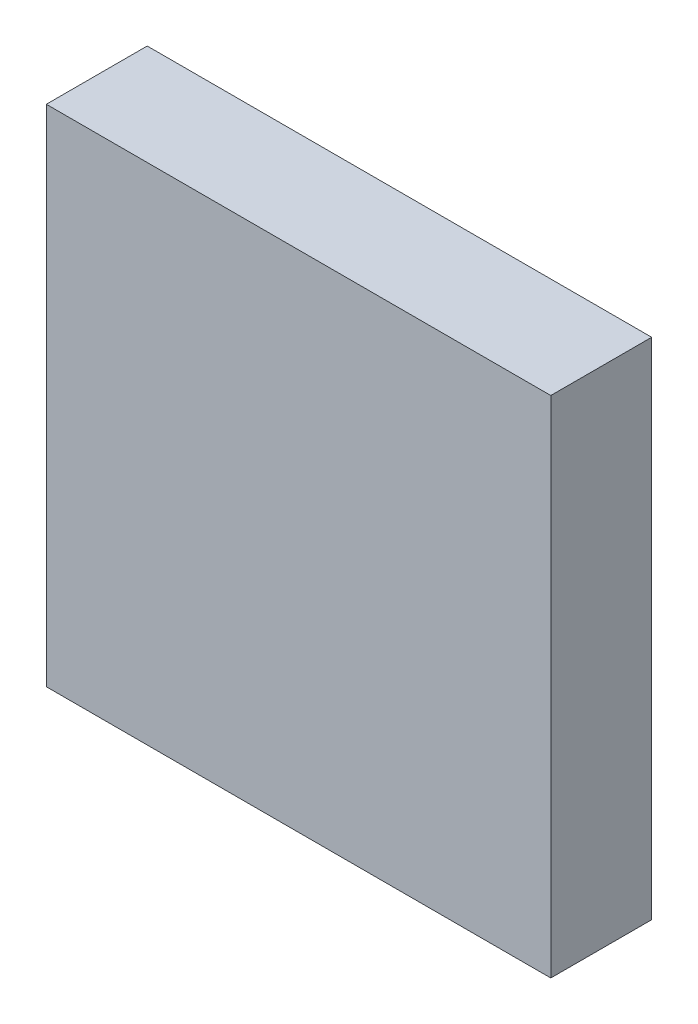
SolidWorks part; units mm, degrees
material "Q235"
ref_plane "Front Plane" through (0, 0, 0) normal (0, 0, 1) x (1, 0, 0)
ref_plane "Top Plane" through (0, 0, 0) normal (0, 1, 0) x (1, 0, 0)
ref_plane "Right Plane" through (0, 0, 0) normal (1, 0, 0) x (0, 0, -1)
sketch "Sketch1" plane through (0, 0, 0) normal (0, 0, 1) x (1, 0, 0)
  line L1 (-40, -40) -> (40, -40)
  line L2 (-40, -40) -> (-40, 40)
  line L3 (-40, 40) -> (40, 40)
  line L4 (40, -40) -> (40, 40)
  line L5 (-40, -40) -> (40, 40) construction
  line L6 (-40, 40) -> (40, -40) construction
  point P0 (0, 0)
  dimension "D1" = 80
  dimension "D2" = 80
extrude "Boss-Extrude1" add sketch "Sketch1" along normal blind 16
chamfer "Chamfer1" [suppressed] distance 15 angle 45
